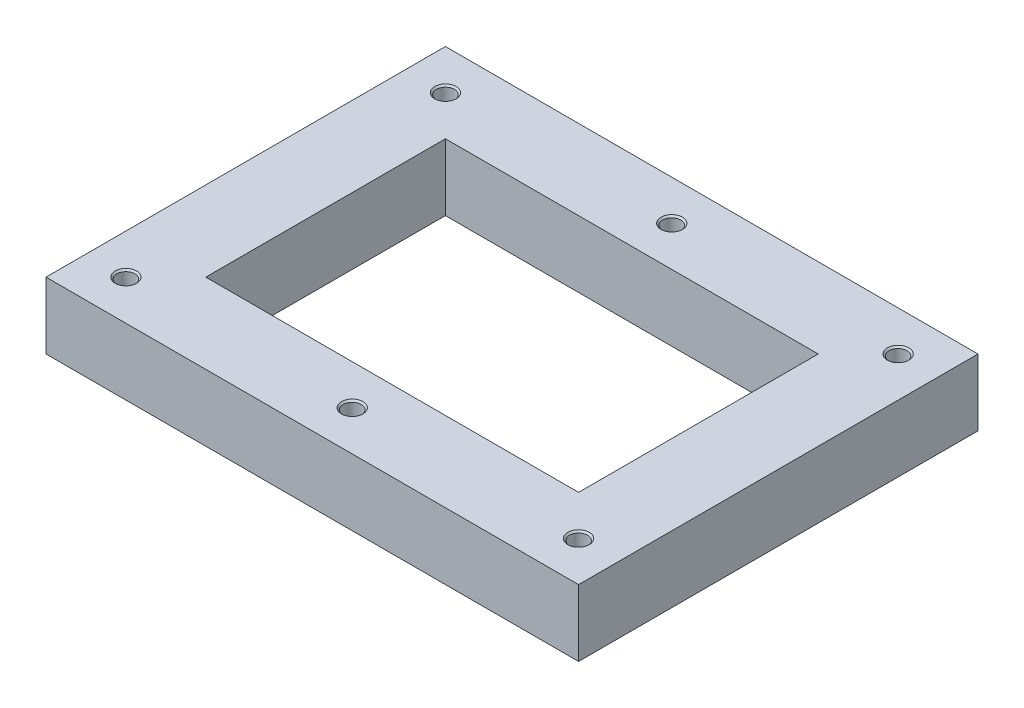
from build123d import *

# Parameters (mm, degrees)
SKETCH_1_W                   = 200
SKETCH_1_H                   = 150
EXTRUDE_1_DEPTH              = 25
HOLE_WIZARD_M8_1_D           = 6.8
HOLE_WIZARD_M8_1_DEPTH       = 17.707073895
HOLE_WIZARD_M8_1_CSINK_D     = 8.05
HOLE_WIZARD_M8_1_CSINK_ANGLE = 90
HOLE_WIZARD_M8_1_TIP         = 2.042926105
CUT_EXTRUDE_1_DEPTH          = 128.47548784
CUT_EXTRUDE_1_DEPTH_BACK     = 128.47548784
SKETCH_5_W                   = 140
SKETCH_5_H                   = 90


with BuildPart() as part:
    # 草图1 → 凸台-拉伸1 (new body)
    with BuildSketch(Plane(origin=(0, 0, 0), x_dir=(1, 0, 0), z_dir=(0, 1, 0))):
        Rectangle(SKETCH_1_W, SKETCH_1_H)
    extrude(amount=EXTRUDE_1_DEPTH)

    # M8 螺纹孔1
    with Locations(Plane(origin=(0, 25, 0), x_dir=(1, 0, 0), z_dir=(0, 1, 0))):
        with Locations((-85, -60), (0, -60), (85, -60), (85, 60), (0, 60), (-85, 60)):
            CounterSinkHole(HOLE_WIZARD_M8_1_D / 2, HOLE_WIZARD_M8_1_CSINK_D / 2, depth=HOLE_WIZARD_M8_1_DEPTH, counter_sink_angle=HOLE_WIZARD_M8_1_CSINK_ANGLE)
            with Locations((0, 0, -(HOLE_WIZARD_M8_1_DEPTH + HOLE_WIZARD_M8_1_TIP / 2))):  # 118° drill point
                Cone(0, HOLE_WIZARD_M8_1_D / 2, HOLE_WIZARD_M8_1_TIP, mode=Mode.SUBTRACT)

    # 草图5 → 切除-拉伸1 (cut, two sides: drawn at the far end of the back side and taken through both)
    with BuildSketch(Plane(origin=(0, 25, 0), x_dir=(1, 0, 0), z_dir=(0, 1, 0)).offset(-CUT_EXTRUDE_1_DEPTH_BACK)):
        Rectangle(SKETCH_5_W, SKETCH_5_H)
    extrude(amount=CUT_EXTRUDE_1_DEPTH + CUT_EXTRUDE_1_DEPTH_BACK, mode=Mode.SUBTRACT)


solid = part.part
